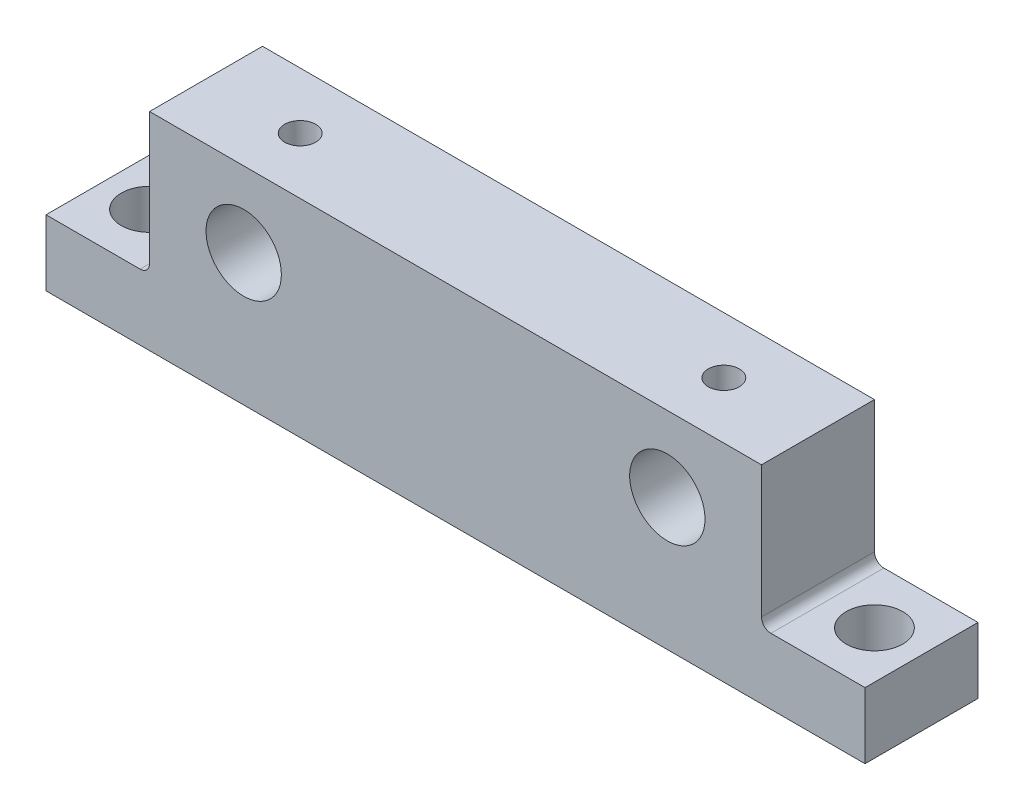
SolidWorks part; units mm, degrees
ref_plane "前视基准面" through (0, 0, 0) normal (0, 0, 1) x (1, 0, 0)
ref_plane "上视基准面" through (0, 0, 0) normal (0, 1, 0) x (1, 0, 0)
ref_plane "右视基准面" through (0, 0, 0) normal (1, 0, 0) x (0, 0, -1)
sketch "草图1" plane through (0, 0, 0) normal (0, 0, 1) x (1, 0, 0)
  line L0 (0, 0) -> (-32.5, 0)
  line L1 (-32.5, 0) -> (-32.5, -15)
  line L2 (-32.5, -15) -> (-43.5, -15)
  line L3 (-43.5, -15) -> (-43.5, -22)
  line L4 (-43.5, -22) -> (43.5, -22)
  line L5 (43.5, -22) -> (43.5, -15)
  line L6 (43.5, -15) -> (32.5, -15)
  line L7 (32.5, -15) -> (32.5, 0)
  line L8 (32.5, 0) -> (0, 0)
  circle A0 centre (-22.5, -8) radius 4
  circle A1 centre (22.5, -8) radius 4
extrude "凸台-拉伸1" add sketch "草图1" along normal mid plane 12
hole_wizard "M4 螺纹孔1" positions "3D草图1" profile "草图2" tap size "M4" standard "GB"
sketch3d "3D草图1"
  line L0 (-32.5, 0, 0) -> (-22.5, 0, 0)
  line L1 (-32.5, 0, 6) -> (-32.5, 0, -6) construction
  point P0 (-22.5, 0, 0)
  dimension "D1" = 10
sketch "草图2" plane through (-22.5, 0, 0) normal (1, 0, 0) x (0, 0, 1)
  line L0 (0, 0) -> (0, 22)
  line L1 (0, 22) -> (1.65, 22)
  line L2 (1.65, 22) -> (1.65, 0)
  line L5 (1.65, 0) -> (0, 0)
  line L11 (0, -6.35) -> (0, 107.95) construction
  dimension "通孔螺纹孔钻头直径" = 3.3
  dimension "通孔螺纹孔钻头深度" = 22
cosmetic thread "孔螺蚊线1" parameters "D2"=4
mirror "镜向1" about plane through (0, 0, 0) normal (1, 0, 0) of "M4 螺纹孔1"
fillet "圆角1" radius 1 2 edges at (32.5, -15, 0) (-32.5, -15, 0)
sketch "草图3" plane through (0, -15, 0) normal (0, 1, 0) x (1, 0, 0)
  line L0 (-43.5, -6) -> (-43.5, 6) construction
  line L1 (43.5, -6) -> (43.5, 6) construction
  circle A0 centre (-38.5, 0) radius 3
  circle A1 centre (38.5, 0) radius 3
  point P4 (0, 0)
  dimension "D1" = 6
  dimension "D2" = 5
  dimension "D3" = 5
extrude "切除-拉伸1" cut sketch "草图3" against normal up to next
equation "\"D7@草图1\"=\"D2@草图1\""
